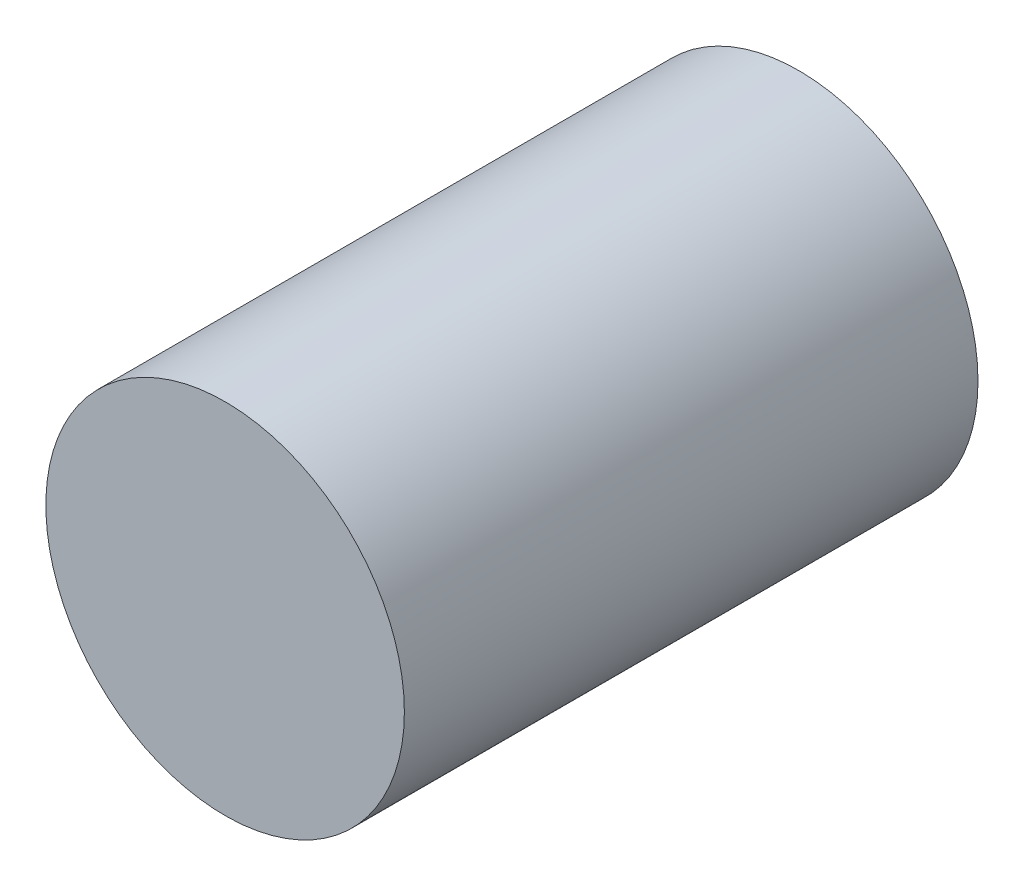
SolidWorks part; units mm, degrees
ref_plane "前视基准面" through (0, 0, 0) normal (0, 0, 1) x (1, 0, 0)
ref_plane "上视基准面" through (0, 0, 0) normal (0, 1, 0) x (1, 0, 0)
ref_plane "右视基准面" through (0, 0, 0) normal (1, 0, 0) x (0, 0, -1)
sketch "草图1" plane through (0, 0, 0) normal (0, 0, 1) x (1, 0, 0)
  circle A0 centre (0, 0) radius 25
  dimension "D1" = 50
extrude "凸台-拉伸1" add sketch "草图1" against normal blind 80
